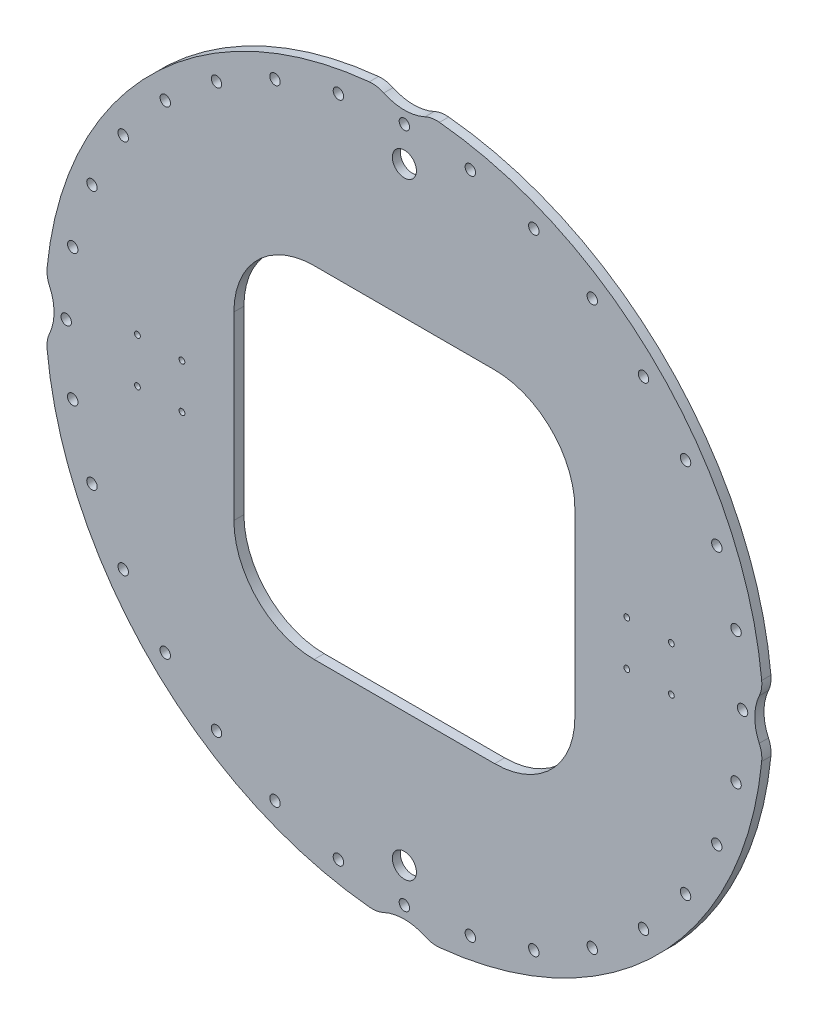
SolidWorks part; units mm, degrees
material "Q235B"
ref_plane "Front Plane" through (0, 0, 0) normal (0, 0, 1) x (1, 0, 0)
ref_plane "Top Plane" through (0, 0, 0) normal (0, 1, 0) x (1, 0, 0)
ref_plane "Right Plane" through (0, 0, 0) normal (1, 0, 0) x (0, 0, -1)
other "Configuration Table"
sketch "Sketch1" plane through (0, 0, 0) normal (0, 0, 1) x (1, 0, 0)
  line L0 (0, 0) -> (0, 263.8214) construction
  line L1 (-225, -425) -> (225, -425)
  line L2 (-425, -225) -> (-425, 225)
  line L3 (-225, 425) -> (225, 425)
  line L4 (425, -225) -> (425, 225)
  line L5 (-425, -425) -> (425, 425) construction
  line L6 (-425, 425) -> (425, -425) construction
  line L7 (554.5, -55.5) -> (665.5, -55.5) construction
  line L8 (554.5, -55.5) -> (554.5, 55.5) construction
  line L9 (554.5, 55.5) -> (665.5, 55.5) construction
  line L10 (665.5, -55.5) -> (665.5, 55.5) construction
  line L11 (554.5, -55.5) -> (665.5, 55.5) construction
  line L12 (554.5, 55.5) -> (665.5, -55.5) construction
  line L13 (0, 0) -> (323.5902, 0) construction
  arc A0 (-87.4722, 890.7152) -> (-890.7152, 87.4722) centre (0, 0) ccw
  circle A1 centre (0, 0) radius 843 construction
  circle A2 centre (0, 843) radius 13
  arc A3 (-51.3105, 884.6139) -> (51.3105, 884.6139) centre (0, 995.85) ccw
  arc A4 (884.6139, 51.3105) -> (884.6139, -51.3105) centre (995.85, 0) ccw
  arc A5 (51.3105, -884.6139) -> (-51.3105, -884.6139) centre (0, -995.85) ccw
  arc A6 (-884.6139, -51.3105) -> (-884.6139, 51.3105) centre (-995.85, 0) ccw
  arc A7 (-425, -225) -> (-225, -425) centre (-225, -225) ccw
  arc A8 (225, -425) -> (425, -225) centre (225, -225) ccw
  arc A9 (425, 225) -> (225, 425) centre (225, 225) ccw
  arc A10 (-225, 425) -> (-425, 225) centre (-225, 225) ccw
  arc A11 (-890.7152, -87.4722) -> (-87.4722, -890.7152) centre (0, 0) ccw
  arc A12 (87.4722, -890.7152) -> (890.7152, -87.4722) centre (0, 0) ccw
  arc A13 (890.7152, 87.4722) -> (87.4722, 890.7152) centre (0, 0) ccw
  circle A14 centre (0, 757) radius 30
  circle A15 centre (554.5, 55.5) radius 7.25
  circle A16 centre (665.5, 55.5) radius 7.25
  circle A17 centre (665.5, -55.5) radius 7.25
  circle A18 centre (554.5, -55.5) radius 7.25
  circle A19 centre (0, -757) radius 30
  arc A20 (-87.4722, 890.7152) -> (-51.3105, 884.6139) centre (-80.6308, 821.0503) cw
  arc A21 (87.4722, 890.7152) -> (51.3105, 884.6139) centre (80.6308, 821.0503) ccw
  arc A22 (884.6139, 51.3105) -> (890.7152, 87.4722) centre (821.0503, 80.6308) ccw
  arc A23 (884.6139, -51.3105) -> (890.7152, -87.4722) centre (821.0503, -80.6308) cw
  arc A24 (51.3105, -884.6139) -> (87.4722, -890.7152) centre (80.6308, -821.0503) ccw
  arc A25 (-51.3105, -884.6139) -> (-87.4722, -890.7152) centre (-80.6308, -821.0503) cw
  arc A26 (-884.6139, -51.3105) -> (-890.7152, -87.4722) centre (-821.0503, -80.6308) ccw
  arc A27 (-884.6139, 51.3105) -> (-890.7152, 87.4722) centre (-821.0503, 80.6308) cw
  circle A28 centre (-665.5, -55.5) radius 7.25
  circle A29 centre (-554.5, -55.5) radius 7.25
  circle A30 centre (-665.5, 55.5) radius 7.25
  circle A31 centre (-554.5, 55.5) radius 7.25
  circle A32 centre (164.4611, 826.802) radius 13
  circle A33 centre (322.6021, 778.8304) radius 13
  circle A34 centre (468.3457, 700.9289) radius 13
  circle A35 centre (596.091, 596.091) radius 13
  circle A36 centre (700.9289, 468.3457) radius 13
  circle A37 centre (778.8304, 322.6021) radius 13
  circle A38 centre (826.802, 164.4611) radius 13
  circle A39 centre (843, 0) radius 13
  circle A40 centre (826.802, -164.4611) radius 13
  circle A41 centre (778.8304, -322.6021) radius 13
  circle A42 centre (700.9289, -468.3457) radius 13
  circle A43 centre (596.091, -596.091) radius 13
  circle A44 centre (468.3457, -700.9289) radius 13
  circle A45 centre (322.6021, -778.8304) radius 13
  circle A46 centre (164.4611, -826.802) radius 13
  circle A47 centre (0, -843) radius 13
  circle A48 centre (-164.4611, -826.802) radius 13
  circle A49 centre (-322.6021, -778.8304) radius 13
  circle A50 centre (-468.3457, -700.9289) radius 13
  circle A51 centre (-596.091, -596.091) radius 13
  circle A52 centre (-700.9289, -468.3457) radius 13
  circle A53 centre (-778.8304, -322.6021) radius 13
  circle A54 centre (-826.802, -164.4611) radius 13
  circle A55 centre (-843, 0) radius 13
  circle A56 centre (-826.802, 164.4611) radius 13
  circle A57 centre (-778.8304, 322.6021) radius 13
  circle A58 centre (-700.9289, 468.3457) radius 13
  circle A59 centre (-596.091, 596.091) radius 13
  circle A60 centre (-468.3457, 700.9289) radius 13
  circle A61 centre (-322.6021, 778.8304) radius 13
  circle A62 centre (-164.4611, 826.802) radius 13
  point P20 (0, 0)
  point P36 (610, 0)
  point P138 (0, 0)
  dimension "D1" = 1790
  dimension "D2" = 1686
  dimension "D3" = 26
  dimension "D5" = 4
  dimension "D8" = 200
  dimension "D10" = 111
  dimension "D14" = 14.5
  dimension "D15" = 70
  dimension "D17" = 60
  dimension "D18" = 122.5
  dimension "D4" = 995.85
  dimension "D6" = 850
  dimension "D7" = 850
  dimension "D9" = 757
  dimension "D11" = 111
  dimension "D12" = 610
  dimension "D13" = 0
  dimension "D16" = 32
extrude "Boss-Extrude1" add sketch "Sketch1" along normal blind 25
sketch "Sketch2" plane through (0, 0, 0) normal (0, 0, -1) x (-1, 0, 0)
  circle A0 centre (0, 0) radius 675
  circle A1 centre (0, 0) radius 870
  dimension "D1" = 1350
  dimension "D2" = 1740
extrude "Cut-Extrude1" cut sketch "Sketch2" against normal blind 5
sketch "Sketch3" plane through (0, 0, 0) normal (0, 0, -1) x (-1, 0, 0)
  circle A0 centre (0, 0) radius 762.2561
  circle A1 centre (0, 0) radius 1126.5479
extrude "Cut-Extrude2" cut sketch "Sketch3" against normal blind 2
